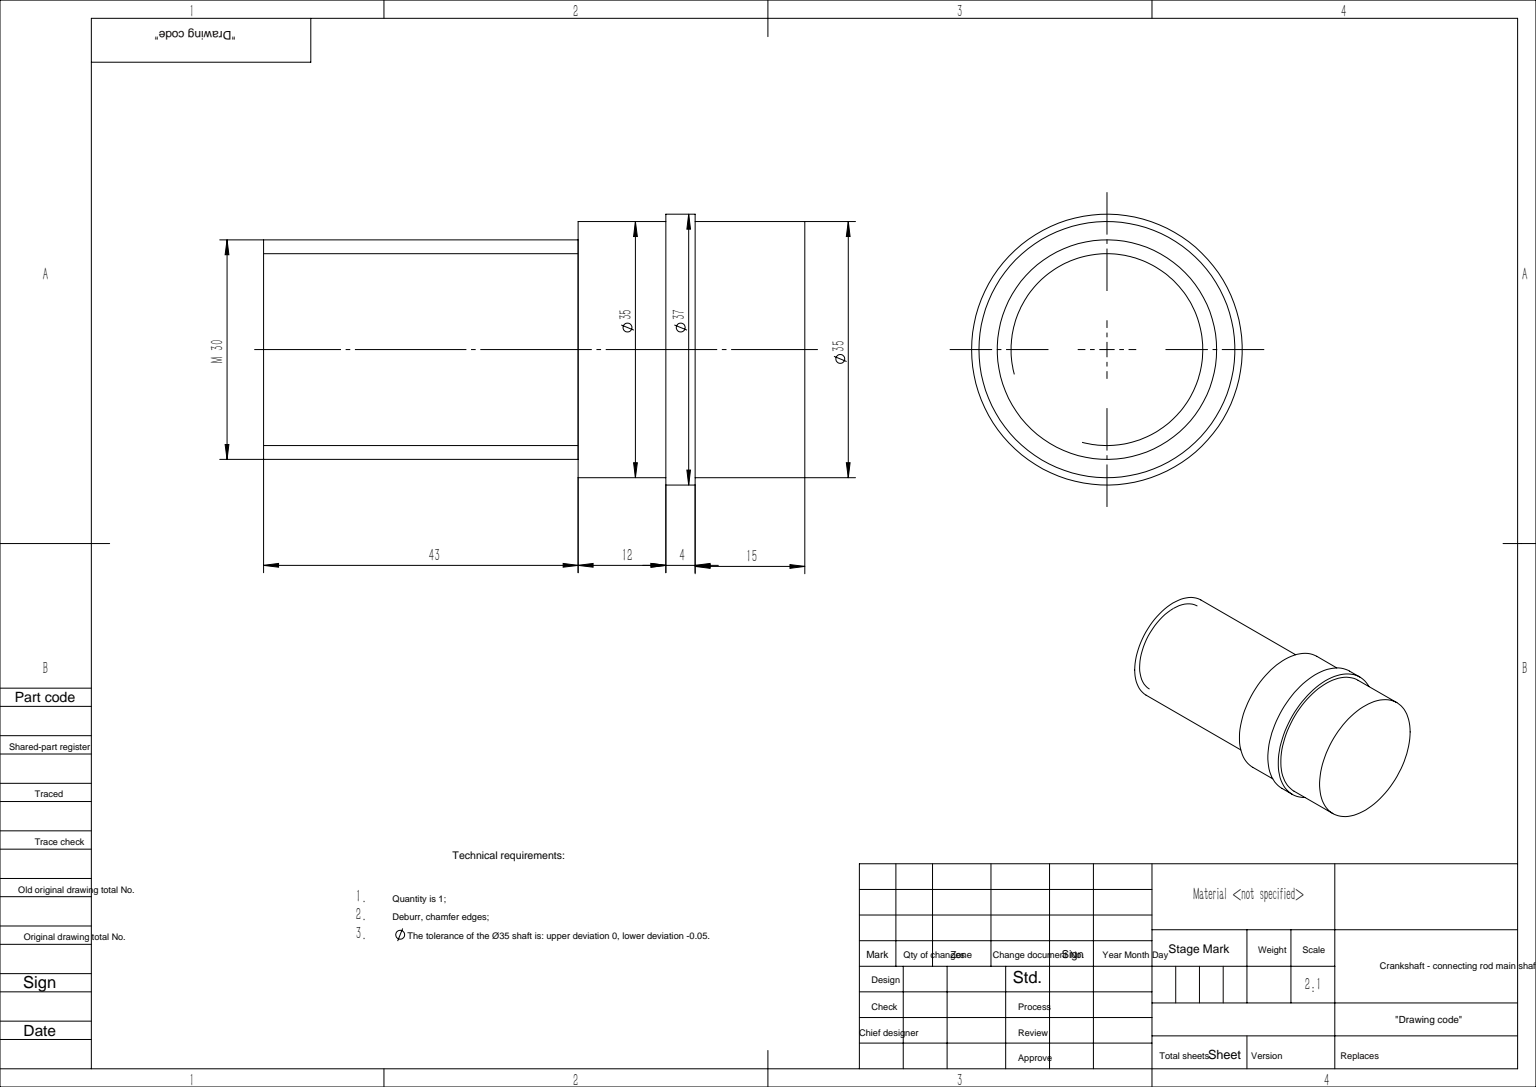
SolidWorks part; units mm, degrees
ref_plane "前视基准面" through (0, 0, 0) normal (0, 0, 1) x (1, 0, 0)
ref_plane "上视基准面" through (0, 0, 0) normal (0, 1, 0) x (1, 0, 0)
ref_plane "右视基准面" through (0, 0, 0) normal (1, 0, 0) x (0, 0, -1)
sketch "草图1" plane through (0, 0, 0) normal (1, 0, 0) x (0, 0, -1)
  circle A0 centre (0, 0) radius 17.5
  dimension "D1" = 35
extrude "凸台-拉伸1" add sketch "草图1" along normal blind 31
sketch "草图2" plane through (0, 0, 0) normal (-1, 0, 0) x (0, 0, 1)
  circle A0 centre (0, 0) radius 15
  dimension "D1" = 30
extrude "凸台-拉伸2" add sketch "草图2" along normal blind 43
cosmetic thread "装饰螺纹线1" parameters "D2"=26.211
ref_plane "基准面1" through (12, 0, 0) normal (1, 0, 0) x (0, 0, -1)
sketch "草图4" plane through (12, 0, 0) normal (1, 0, 0) x (0, 0, -1)
  circle A0 centre (0, 0) radius 18.5
  dimension "D1" = 37
extrude "凸台-拉伸3" add sketch "草图4" along normal blind 4
